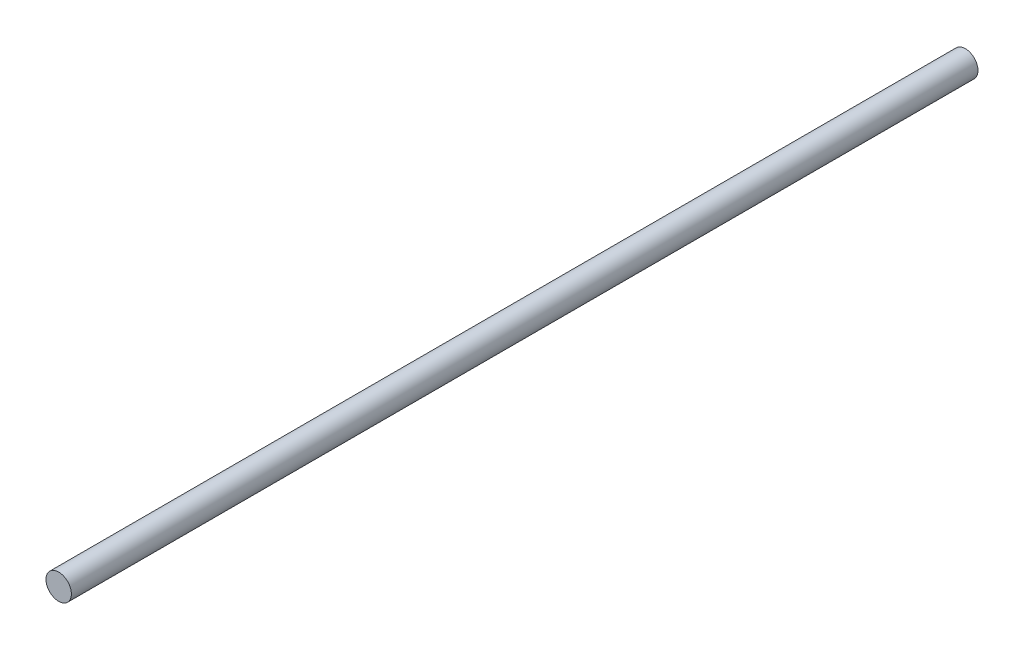
SolidWorks part; units mm, degrees
ref_plane "Front Plane" through (0, 0, 0) normal (0, 0, 1) x (1, 0, 0)
ref_plane "Top Plane" through (0, 0, 0) normal (0, 1, 0) x (1, 0, 0)
ref_plane "Right Plane" through (0, 0, 0) normal (1, 0, 0) x (0, 0, -1)
other "Configuration Table"
sketch "Sketch1" plane through (0, 0, 0) normal (0, 0, 1) x (1, 0, 0)
  circle A0 centre (0, 0) radius 2.5
  dimension "D1" = 5
extrude "Boss-Extrude1" add sketch "Sketch1" along normal blind 178.5
